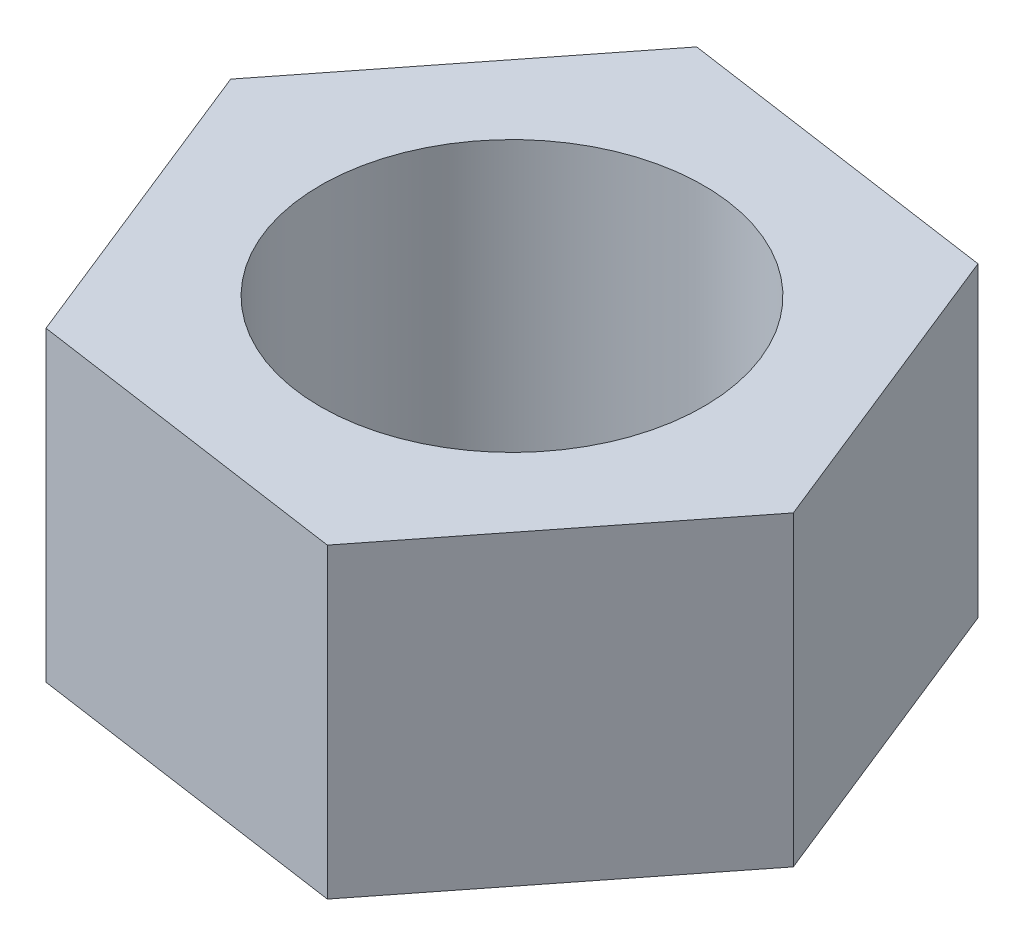
SolidWorks part; units mm, degrees
ref_plane "Front Plane" through (0, 0, 0) normal (0, 0, 1) x (1, 0, 0)
ref_plane "Top Plane" through (0, 0, 0) normal (0, 1, 0) x (1, 0, 0)
ref_plane "Right Plane" through (0, 0, 0) normal (1, 0, 0) x (0, 0, -1)
sketch "Sketch1" plane through (0, 0, 0) normal (0, 1, 0) x (1, 0, 0)
  line L1 (2.1409, 2.7233) -> (-1.288, 3.2157)
  line L2 (-1.288, 3.2157) -> (-3.4289, 0.4924)
  line L3 (-3.4289, 0.4924) -> (-2.1409, -2.7233)
  line L4 (-2.1409, -2.7233) -> (1.288, -3.2157)
  line L5 (1.288, -3.2157) -> (3.4289, -0.4924)
  line L6 (3.4289, -0.4924) -> (2.1409, 2.7233)
  circle A0 centre (0, 0) radius 3 construction
  circle A1 centre (0, 0) radius 2
  dimension "D1" = 4
  dimension "D2" = 6
extrude "Boss-Extrude1" add sketch "Sketch1" along normal blind 3.2
